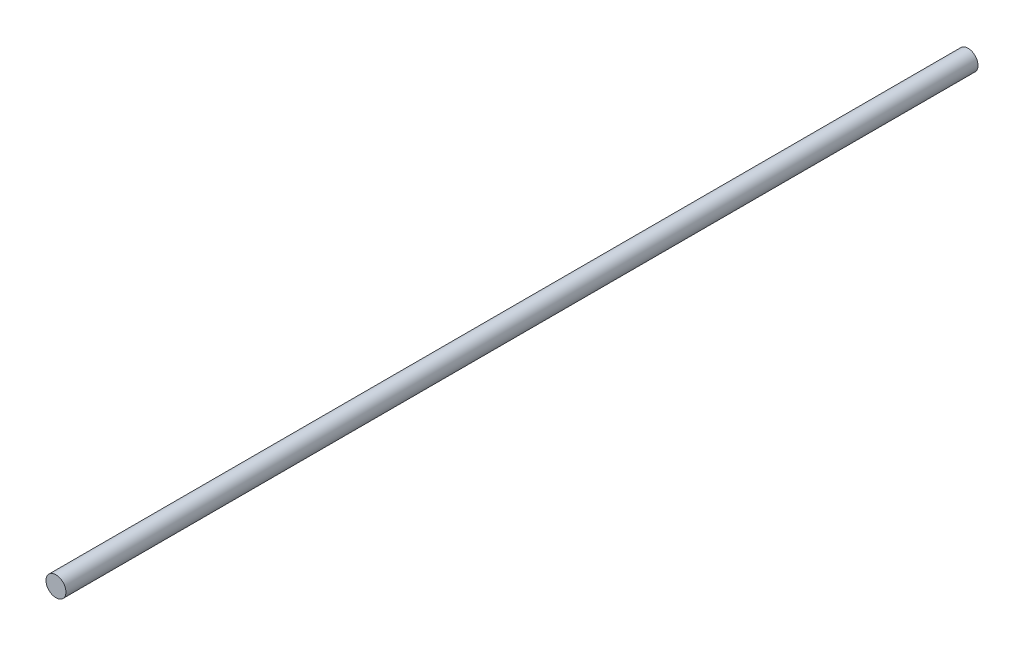
SolidWorks part; units mm, degrees
ref_plane "Front Plane" through (0, 0, 0) normal (0, 0, 1) x (1, 0, 0)
ref_plane "Top Plane" through (0, 0, 0) normal (0, 1, 0) x (1, 0, 0)
ref_plane "Right Plane" through (0, 0, 0) normal (1, 0, 0) x (0, 0, -1)
other "Configuration Table"
sketch "Sketch1" plane through (0, 0, 0) normal (0, 0, 1) x (1, 0, 0)
  circle A0 centre (0, 0) radius 1.44
  dimension "D1" = 2.88
extrude "Boss-Extrude1" add sketch "Sketch1" along normal blind 131.6
